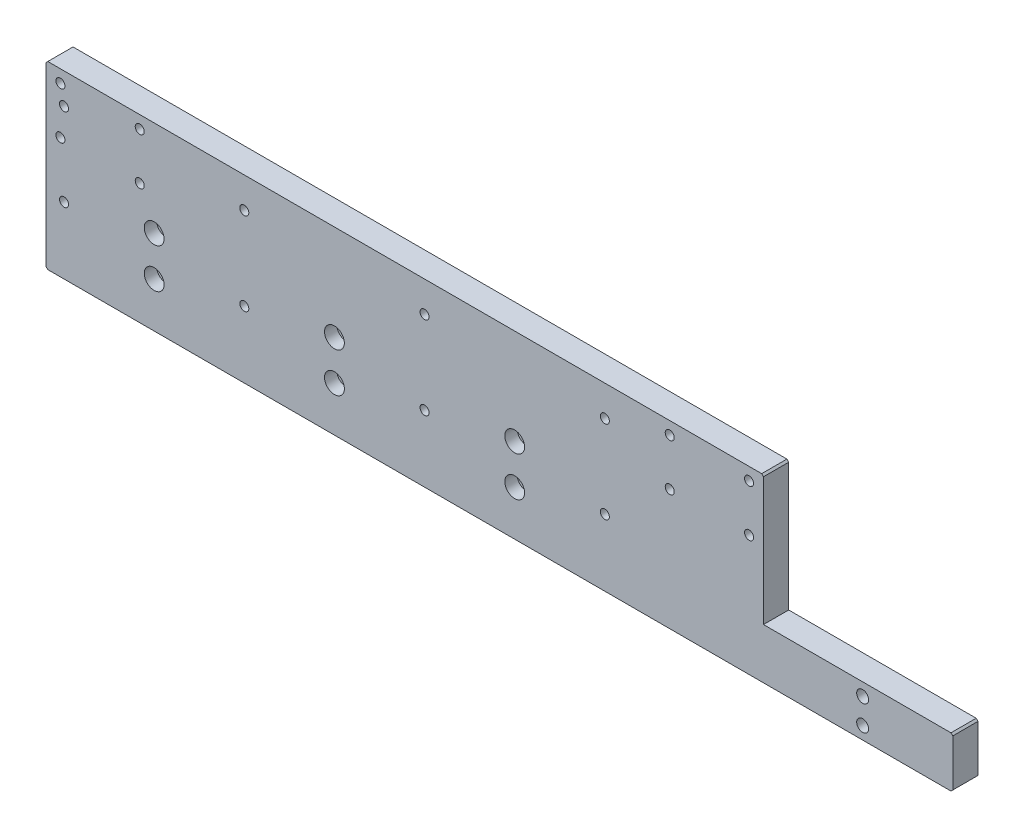
SolidWorks part; units mm, degrees
material "AL6061"
ref_plane "Front Plane" through (0, 0, 0) normal (0, 0, 1) x (1, 0, 0)
ref_plane "Top Plane" through (0, 0, 0) normal (0, 1, 0) x (1, 0, 0)
ref_plane "Right Plane" through (0, 0, 0) normal (1, 0, 0) x (0, 0, -1)
sketch "Sketch1" plane through (0, 0, 0) normal (0, 0, 1) x (1, 0, 0)
  line L1 (-199, -50) -> (199, -50)
  line L2 (-199, -50) -> (-199, 50)
  line L3 (-199, 50) -> (199, 50)
  line L4 (199, -50) -> (199, 50)
  line L5 (-199, -50) -> (199, 50) construction
  line L6 (-199, 50) -> (199, -50) construction
  point P0 (0, 0)
  dimension "D1" = 100
  dimension "D2" = 398
extrude "Boss-Extrude1" add sketch "Sketch1" along normal mid plane 14
sketch "Sketch2" plane through (199, 0, 0) normal (1, 0, 0) x (0, 0, -1)
  line L0 (7, -50) -> (7, 50) construction
  line L1 (-7, -50) -> (7, -50)
  line L2 (-7, -50) -> (-7, -22)
  line L3 (-7, -22) -> (7, -22)
  line L4 (7, -50) -> (7, -22)
  dimension "D1" = 28
extrude "Boss-Extrude2" add sketch "Sketch2" along normal blind 105
hole_wizard "M6 Clearance Hole1" positions "Sketch3" profile "Sketch4" hole size "M6" standard "GB" end condition through all
sketch "Sketch3" plane through (0, 0, -7) normal (0, 0, -1) x (-1, 0, 0)
  line L0 (-343.9062, -36) -> (-224.1109, -36) construction
  line L1 (-358.066, -29) -> (-131.9169, -29) construction
  line L5 (-304, -22) -> (-199, -22) construction
  line L6 (-304, -50) -> (-304, -22) construction
  point P6 (-254, -29)
  point P12 (-254, -43)
  dimension "D1" = 7
  dimension "D2" = 50
  dimension "D3" = 14
sketch "Sketch4" plane through (254, -43, -7) normal (1, 0, 0) x (0, 1, 0)
  line L0 (0, 0) -> (0, 14)
  line L1 (0, 14) -> (3.3, 14)
  line L2 (3.3, 14) -> (3.3, 0)
  line L5 (3.3, 0) -> (0, 0)
  line L11 (0, -6.35) -> (0, 107.95) construction
  dimension "通孔孔直径" = 6.6
  dimension "通孔孔深度" = 14
hole_wizard "M6 Tapped Hole1" positions "Sketch5" profile "Sketch6" tap size "M6" standard "GB" end condition through all
sketch "Sketch5" plane through (0, 0, 7) normal (0, 0, 1) x (1, 0, 0)
  line L0 (-189, 70.679) -> (-189, -92.1145) construction
  line L2 (199, 50) -> (-199, 50) construction
  line L3 (-189, -13) -> (-89, -13) construction
  line L4 (304, -22) -> (304, -50) construction
  point P7 (-189, 33)
  point P9 (-189, -13)
  point P20 (-89, 33)
  point P21 (-89, -13)
  point P22 (11, 33)
  point P23 (11, -13)
  point P24 (111, 33)
  point P25 (111, -13)
  dimension "D1" = 46
  dimension "D2" = 193
  dimension "D3" = 17
  dimension "D5" = 100
  dimension "D4" = 4
sketch "Sketch6" plane through (111, -13, 7) normal (1, 0, 0) x (0, -1, 0)
  line L0 (0, 0) -> (0, 14)
  line L1 (0, 14) -> (2.5, 14)
  line L2 (2.5, 14) -> (2.5, 0)
  line L5 (2.5, 0) -> (0, 0)
  line L11 (0, -6.35) -> (0, 107.95) construction
  dimension "通孔螺纹孔钻头直径" = 5
  dimension "通孔螺纹孔钻头深度" = 14
cosmetic thread "Cosmetic Thread1" parameters "D2"=6
cosmetic thread "Cosmetic Thread2" parameters "D2"=6
cosmetic thread "Cosmetic Thread3" parameters "D2"=6
cosmetic thread "Cosmetic Thread4" parameters "D2"=6
cosmetic thread "Cosmetic Thread5" parameters "D2"=6
cosmetic thread "Cosmetic Thread6" parameters "D2"=6
cosmetic thread "Cosmetic Thread7" parameters "D2"=6
cosmetic thread "Cosmetic Thread8" parameters "D2"=6
hole_wizard "Hole Size per Socket Head Cap Screw Type1" positions "Sketch7" profile "Sketch8" counterbore size "M6" standard "GB" end condition through all
sketch "Sketch7" plane through (0, 0, 7) normal (0, 0, 1) x (1, 0, 0)
  line L0 (61, 70.4796) -> (61, -119.0292) construction
  line L1 (-199, -50) -> (304, -50) construction
  line L2 (61, -3) -> (-39, -3) construction
  circle A0 centre (111, 33) radius 2.5 construction
  circle A1 centre (11, 33) radius 2.5 construction
  point P10 (61, -25)
  point P12 (61, -3)
  point P21 (-39, -25)
  point P22 (-39, -3)
  point P23 (-139, -25)
  point P24 (-139, -3)
  dimension "D1" = 22
  dimension "D2" = 25
  dimension "D4" = 100
  dimension "D3" = 3
sketch "Sketch8" plane through (-139, -3, 7) normal (1, 0, 0) x (0, -1, 0)
  line L0 (0, 0) -> (0, 14)
  line L1 (0, 14) -> (3.3, 14)
  line L3 (3.3, 14) -> (3.3, 6.8)
  line L4 (3.3, 6.8) -> (5.5, 6.8)
  line L5 (5.5, 6.8) -> (5.5, 0)
  line L7 (5.5, 0) -> (0, 0)
  line L11 (0, -6.35) -> (0, 107.95) construction
  dimension "通孔孔直径" = 6.6
  dimension "通孔孔深度" = 14
  dimension "柱形沉头孔直径" = 11
  dimension "柱形沉头孔深度" = 6.8
hole_wizard "M6 Tapped Hole2" positions "Sketch9" profile "Sketch10" tap size "M6" standard "GB" end condition through all
sketch "Sketch9" plane through (0, 0, -7) normal (0, 0, -1) x (-1, 0, 0)
  line L1 (-191, 43) -> (-147, 43)
  line L2 (-191, 43) -> (-191, 17)
  line L3 (-191, 17) -> (-147, 17)
  line L4 (-147, 43) -> (-147, 17)
  line L5 (0, 50) -> (0, -120.0821) construction
  line L6 (-199, 50) -> (199, 50) construction
  line L7 (147, 43) -> (147, 17)
  line L8 (191, 17) -> (147, 17)
  line L9 (191, 43) -> (191, 17)
  line L10 (191, 43) -> (147, 43)
  line L11 (-199, -22) -> (-199, 50) construction
  point P1 (-191, 43)
  point P2 (-147, 17)
  point P133 (-191, 17)
  point P134 (-147, 43)
  point P154 (147, 43)
  point P155 (191, 17)
  point P156 (147, 17)
  point P157 (191, 43)
  dimension "D1" = 8
  dimension "D2" = 7
  dimension "D3" = 44
  dimension "D4" = 26
sketch "Sketch10" plane through (191, 43, -7) normal (1, 0, 0) x (0, 1, 0)
  line L0 (0, 0) -> (0, 14)
  line L1 (0, 14) -> (2.5, 14)
  line L2 (2.5, 14) -> (2.5, 0)
  line L5 (2.5, 0) -> (0, 0)
  line L11 (0, -6.35) -> (0, 107.95) construction
  dimension "通孔螺纹孔钻头直径" = 5
  dimension "通孔螺纹孔钻头深度" = 14
cosmetic thread "Cosmetic Thread9" parameters "D2"=6
cosmetic thread "Cosmetic Thread10" parameters "D2"=6
cosmetic thread "Cosmetic Thread11" parameters "D2"=6
cosmetic thread "Cosmetic Thread12" parameters "D2"=6
cosmetic thread "Cosmetic Thread13" parameters "D2"=6
cosmetic thread "Cosmetic Thread14" parameters "D2"=6
cosmetic thread "Cosmetic Thread15" parameters "D2"=6
cosmetic thread "Cosmetic Thread16" parameters "D2"=6
hole_wizard "M6 Tapped Hole3" positions "Sketch11" profile "Sketch12" tap size "M6" standard "GB"
sketch "Sketch11" plane through (0, -50, 0) normal (0, -1, 0) x (-1, 0, 0)
  line L0 (0, 0) -> (-354.5568, 0) construction
  line L1 (199, -7) -> (199, 7) construction
  line L2 (189, 0) -> (89, 0) construction
  point P8 (189, 0)
  point P18 (89, 0)
  point P19 (-11, 0)
  point P20 (-111, 0)
  point P21 (-211, 0)
  point P26 (-291, 0)
  dimension "D1" = 10
  dimension "D3" = 100
  dimension "D4" = 80
  dimension "D2" = 5
sketch "Sketch12" plane through (291, -50, 0) normal (1, 0, 0) x (0, 0, -1)
  line L0 (0, 0) -> (0, 16.5022)
  line L1 (0, 16.5022) -> (2.5, 15)
  line L2 (2.5, 15) -> (2.5, 0)
  line L5 (2.5, 0) -> (0, 0)
  line L10 (0, 16.5022) -> (-2.5, 15) construction
  line L11 (0, -6.35) -> (0, 107.95) construction
  dimension "螺纹孔钻头直径" = 5
  dimension "螺纹孔钻头深度" = 15
  dimension "导头角度" = 118
cosmetic thread "Cosmetic Thread17" parameters "D1"=12, "D2"=6
cosmetic thread "Cosmetic Thread18" parameters "D1"=12, "D2"=6
cosmetic thread "Cosmetic Thread19" parameters "D1"=12, "D2"=6
cosmetic thread "Cosmetic Thread20" parameters "D1"=12, "D2"=6
cosmetic thread "Cosmetic Thread21" parameters "D1"=12, "D2"=6
cosmetic thread "Cosmetic Thread22" parameters "D1"=12, "D2"=6
chamfer "Chamfer1" distance 1 angle 45 5 edges at (199, 50, 0) (304, -22, 0) (304, -50, 0) (-199, -50, 0) (-199, 50, 0)
